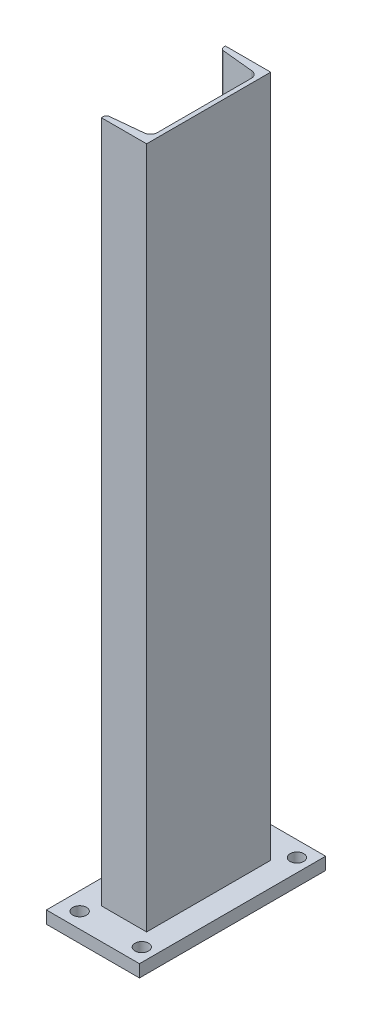
SolidWorks part; units mm, degrees
material "Q235B"
ref_plane "Front" through (0, 0, 0) normal (0, 0, 1) x (1, 0, 0)
ref_plane "Top" through (0, 0, 0) normal (0, 1, 0) x (1, 0, 0)
ref_plane "Right" through (0, 0, 0) normal (1, 0, 0) x (0, 0, -1)
sketch "草图1" plane through (0, 0, 0) normal (0, 0, 1) x (1, 0, 0)
  line L0 (0, 588.7097) -> (0, -511.2903)
  dimension "D1" = 1100
other "Structural Member1"
ref_plane "Plane1" through (0, 588.7097, 0) normal (0, -1, 0) x (1, 0, 0)
sketch "Sketch1" plane through (0, 588.7097, 0) normal (0, -1, 0) x (1, 0, 0)
  line L0 (0, 0) -> (0, -200)
  line L1 (0, -200) -> (-73, -200)
  line L2 (0, -100) -> (-73, -100) construction
  line L3 (-7, -175.7451) -> (-7, -24.2549)
  line L4 (-16.9055, -186.6905) -> (-68.0473, -191.8047)
  line L5 (-73, -197.2774) -> (-73, -200)
  line L6 (-73, -200) -> (0, -192.7) construction
  line L7 (-73, -197.2774) -> (-7, -197.2774) construction
  line L8 (-73, -2.7226) -> (-73, -197.2774) construction
  line L9 (-73, -2.7226) -> (-73, 0)
  line L10 (0, 0) -> (-73, 0)
  line L11 (-16.9055, -13.3095) -> (-68.0473, -8.1953)
  line L12 (-7, -197.2774) -> (-7, -175.7451) construction
  line L13 (-40, -189) -> (-40, -200) construction
  arc A0 (-7, -175.7451) -> (-16.9055, -186.6905) centre (-18, -175.7451) cw
  arc A1 (-16.9055, -13.3095) -> (-7, -24.2549) centre (-18, -24.2549) cw
  arc A2 (-68.0473, -191.8047) -> (-73, -197.2774) centre (-67.5, -197.2774) ccw
  arc A3 (-73, -2.7226) -> (-68.0473, -8.1953) centre (-67.5, -2.7226) ccw
  point P2 (-36.5, 0)
  point P5 (-7, -100)
  point P10 (-36.5, -200)
  point P20 (-7, -14.3)
  point P26 (-73, -7.7)
  point P27 (-40, -197.2774)
  point P29 (0, 0)
  dimension "r" = 11
  dimension "r1" = 5.5
  dimension "h" = 200
  dimension "b" = 73
  dimension "d" = 7
  dimension "t" = 11
  dimension "a" = 7.3
sketch "Sketch3" plane through (0, -511.2903, 0) normal (0, -1, 0) x (1, 0, 0)
  line L0 (0, -100) -> (-78.8326, -100) construction
  line L1 (38.5, -250) -> (-111.5, -250)
  line L2 (38.5, -250) -> (38.5, 50)
  line L3 (38.5, 50) -> (-111.5, 50)
  line L4 (-111.5, -250) -> (-111.5, 50)
  line L5 (-36.5, 50) -> (-36.5, -250) construction
  line L6 (38.5, -100) -> (-111.5, -100) construction
  line L7 (0, -200) -> (0, 0) construction
  line L8 (-36.5, 0) -> (-36.5, -200) construction
  line L9 (0, 0) -> (-73, 0) construction
  line L10 (-73, -200) -> (0, -200) construction
  point P0 (-36.5, -100)
  dimension "D1" = 150
  dimension "D2" = 300
extrude "Boss-Extrude1" add sketch "Sketch3" along normal blind 20 separate body
hole_wizard "Ø22.0 (22) Hole1" positions "Sketch5" profile "Sketch4" hole size "Ø22.0" standard "GB" end condition up to next
sketch "Sketch5" plane through (0, -511.2903, 0) normal (0, 1, 0) x (1, 0, 0)
  line L0 (-36.5, 250) -> (-36.5, 138.4474) construction
  line L1 (-111.5, 250) -> (38.5, 250) construction
  point P0 (-82.7665, 225)
  point P2 (17.2335, 225)
  dimension "D1" = 100
  dimension "D2" = 25
sketch "Sketch4" plane through (-82.7665, -511.2903, -225) normal (1, 0, 0) x (0, 0, 1)
  line L0 (0, 0) -> (0, 20.001)
  line L1 (0, 20.001) -> (11, 20.001)
  line L2 (11, 20.001) -> (11, 0)
  line L5 (11, 0) -> (0, 0)
  line L11 (0, -6.35) -> (0, 107.95) construction
  dimension "通孔孔直径" = 22
  dimension "通孔孔深度" = 20.001
ref_plane "Plane2" through (0, 0, -100) normal (0, 0, -1) x (-1, 0, 0)
mirror "Mirror1" about plane through (0, 0, -100) normal (0, 0, -1) of "Ø22.0 (22) Hole1"
equation "\"零件重量\"= IIF ( \"SW-质量\" > 100 , int ( \"SW-质量\" ) , \"SW-质量\" )"
